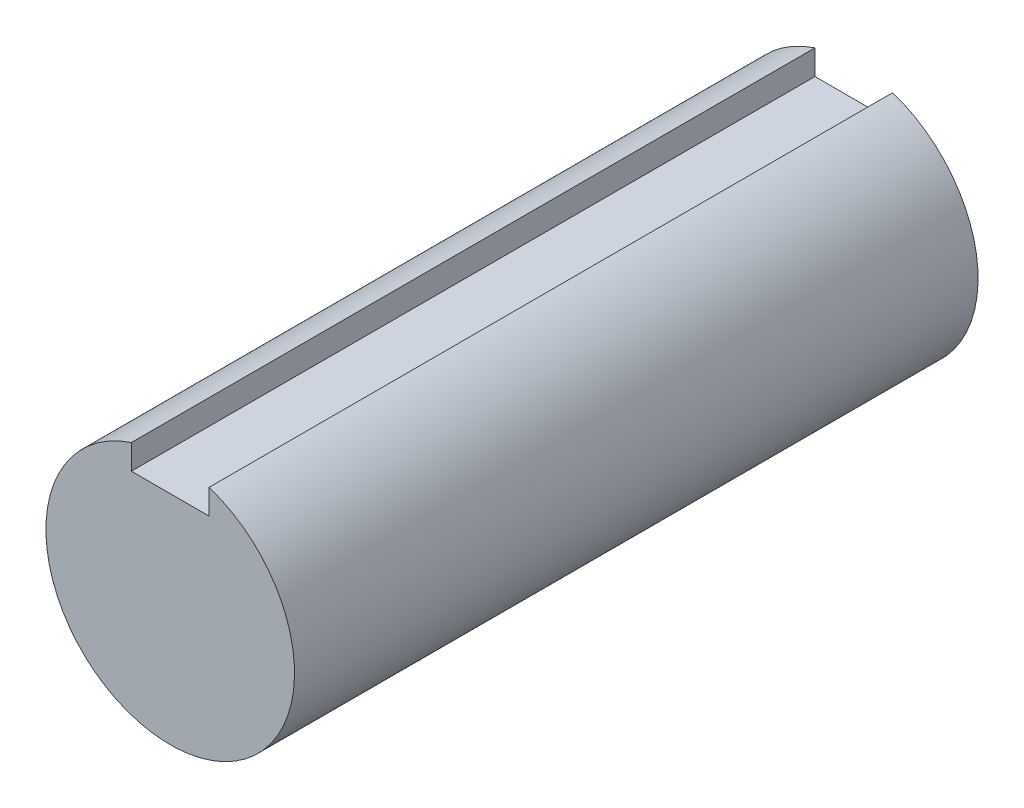
SolidWorks part; units mm, degrees
ref_plane "Front Plane" through (0, 0, 0) normal (0, 0, 1) x (1, 0, 0)
ref_plane "Top Plane" through (0, 0, 0) normal (0, 1, 0) x (1, 0, 0)
ref_plane "Right Plane" through (0, 0, 0) normal (1, 0, 0) x (0, 0, -1)
other "Configuration Table"
sketch "Sketch1" plane through (0, 0, 0) normal (0, 0, 1) x (1, 0, 0)
  line L0 (-271.5, 6) -> (-271.5, 7.5993)
  line L1 (-271.5, 6) -> (-276.5, 6)
  line L3 (-276.5, 6) -> (-276.5, 7.5993)
  circle A0 centre (-274, 0) radius 8 construction
  arc A1 (-276.5, 7.5993) -> (-271.5, 7.5993) centre (-274, 0) ccw
extrude "Boss-Extrude1" add sketch "Sketch1" against normal up to surface (44 mm away)
